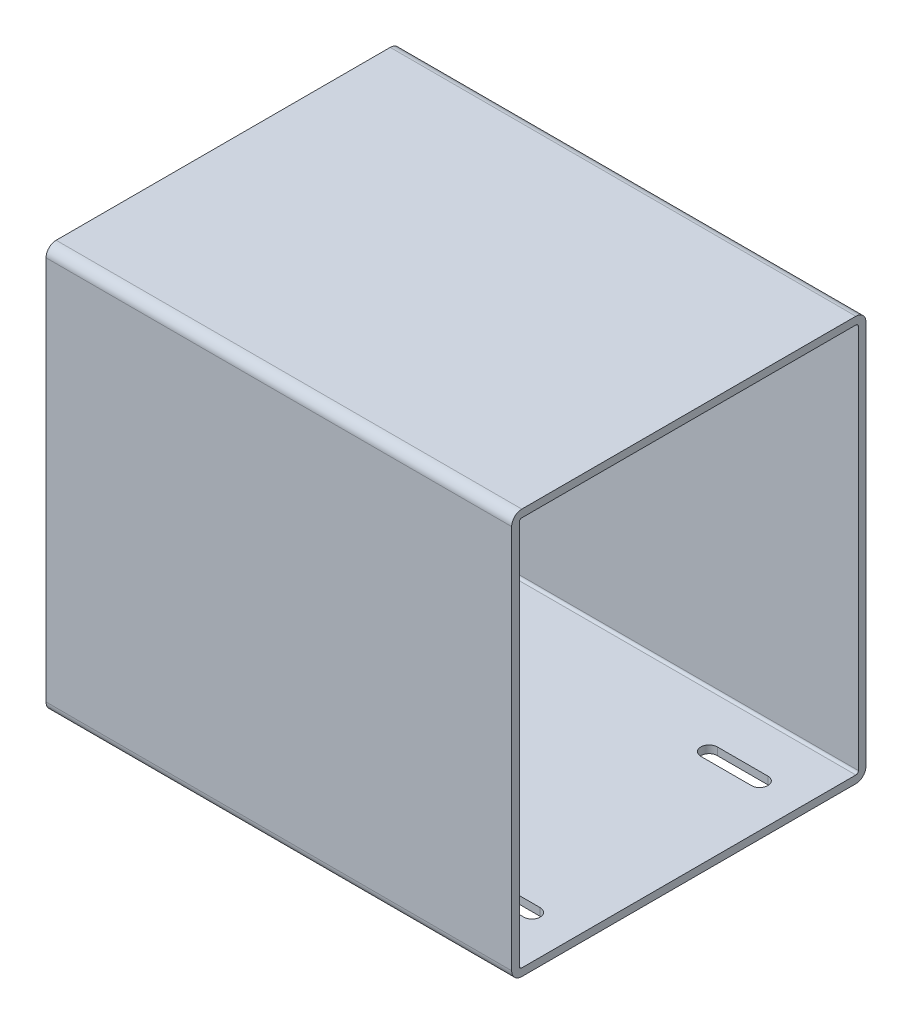
SolidWorks part; units mm, degrees
material "Q235-A "
ref_plane "前视基准面" through (0, 0, 0) normal (0, 0, 1) x (1, 0, 0)
ref_plane "上视基准面" through (0, 0, 0) normal (0, 1, 0) x (1, 0, 0)
ref_plane "右视基准面" through (0, 0, 0) normal (1, 0, 0) x (0, 0, -1)
sketch "草图2" plane through (0, 0, 0) normal (1, 0, 0) x (0, 0, -1)
  line L0 (-67, 77) -> (67, 77)
  line L1 (-70, 80) -> (70, 80)
  line L2 (-70, 80) -> (-70, -80)
  line L3 (-70, -80) -> (70, -80)
  line L4 (70, 80) -> (70, -80)
  line L5 (-70, 80) -> (70, -80) construction
  line L6 (-70, -80) -> (70, 80) construction
  line L7 (67, 77) -> (67, -77)
  line L8 (-67, -77) -> (67, -77)
  line L9 (-67, 77) -> (-67, -77)
  point P0 (0, 0)
  dimension "D2" = 140
  dimension "D3" = 160
  dimension "D1" = 3
extrude "凸台-拉伸1" add sketch "草图2" along normal blind 150 and the other way blind 34
sketch "草图3" plane through (0, -77, 0) normal (0, 1, 0) x (1, 0, 0)
  line L0 (-17, 45) -> (3, 45) construction
  line L1 (-17, 48.25) -> (3, 48.25)
  line L2 (-17, 41.75) -> (3, 41.75)
  line L3 (150, 0) -> (-34, 0) construction
  line L5 (58, 70) -> (58, -70) construction
  line L6 (-34, 70) -> (150, 70) construction
  line L7 (-34, -70) -> (150, -70) construction
  line L8 (150, 70) -> (150, -70) construction
  line L9 (-34, 70) -> (-34, -70) construction
  line L10 (-17, -45) -> (3, -45) construction
  line L11 (-17, -48.25) -> (3, -48.25)
  line L12 (-17, -41.75) -> (3, -41.75)
  line L13 (133, 45) -> (113, 45) construction
  line L14 (133, 48.25) -> (113, 48.25)
  line L15 (133, 41.75) -> (113, 41.75)
  line L16 (133, -45) -> (113, -45) construction
  line L17 (133, -48.25) -> (113, -48.25)
  line L18 (133, -41.75) -> (113, -41.75)
  arc A0 (-17, 48.25) -> (-17, 41.75) centre (-17, 45) ccw
  arc A1 (3, 41.75) -> (3, 48.25) centre (3, 45) ccw
  arc A2 (-17, -48.25) -> (-17, -41.75) centre (-17, -45) cw
  arc A3 (3, -41.75) -> (3, -48.25) centre (3, -45) cw
  arc A4 (133, 48.25) -> (133, 41.75) centre (133, 45) cw
  arc A5 (113, 41.75) -> (113, 48.25) centre (113, 45) cw
  arc A6 (133, -48.25) -> (133, -41.75) centre (133, -45) ccw
  arc A7 (113, -41.75) -> (113, -48.25) centre (113, -45) ccw
  point P2 (-7, 45)
  point P22 (-7, -45)
  point P29 (123, 45)
  point P36 (123, -45)
  dimension "D4" = 3.25
  dimension "D1" = 90
  dimension "D2" = 130
  dimension "D3" = 20
extrude "切除-拉伸1" cut sketch "草图3" against normal blind 10
fillet "圆角1" radius 1 4 edges at (58, 77, -67) (58, 77, 67) (58, -77, 67) (58, -77, -67)
fillet "圆角2" radius 4 4 edges at (58, -80, 70) (58, -80, -70) (58, 80, -70) (58, 80, 70)
